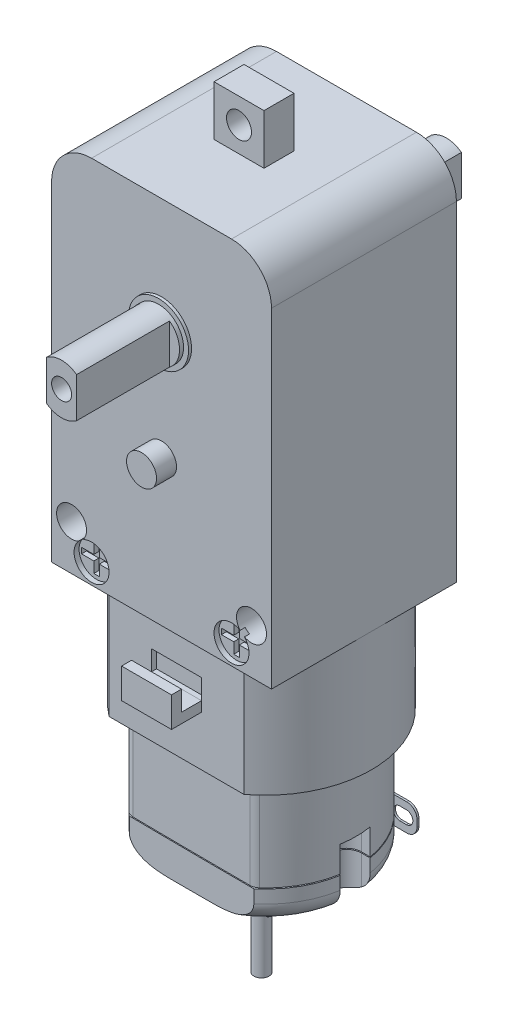
SolidWorks part; units mm, degrees
ref_plane "Front Plane" through (0, 0, 0) normal (0, 0, 1) x (1, 0, 0)
ref_plane "Top Plane" through (0, 0, 0) normal (0, 1, 0) x (1, 0, 0)
ref_plane "Right Plane" through (0, 0, 0) normal (1, 0, 0) x (0, 0, -1)
sketch "Sketch1" plane through (0, 0, 0) normal (0, 0, 1) x (1, 0, 0)
  line L1 (-11, 24.5) -> (11, 24.5)
  line L2 (-11, 24.5) -> (-11, -24.5)
  line L3 (-11, -24.5) -> (11, -24.5)
  line L4 (11, 24.5) -> (11, -24.5)
  line L5 (-11, 24.5) -> (11, -24.5) construction
  line L6 (-11, -24.5) -> (11, 24.5) construction
  point P0 (0, 0)
  dimension "D1" = 22
  dimension "D2" = 49
extrude "Boss-Extrude1" add sketch "Sketch1" along normal mid plane 18.5
sketch "Sketch2" plane through (0, 0, 0) normal (0, 0, 1) x (1, 0, 0)
  line L0 (11, 24.5) -> (-11, 24.5) construction
  line L1 (-2.5, 29.5) -> (2.5, 29.5)
  line L2 (-2.5, 29.5) -> (-2.5, 19.5)
  line L3 (-2.5, 19.5) -> (2.5, 19.5)
  line L4 (2.5, 29.5) -> (2.5, 19.5)
  line L5 (-2.5, 29.5) -> (2.5, 19.5) construction
  line L6 (-2.5, 19.5) -> (2.5, 29.5) construction
  line L7 (-2.5, 29.5) -> (2.5, 24.5) construction
  circle A0 centre (0, 27) radius 1.25
  point P0 (0, 24.5)
  dimension "D3" = 2.5
  dimension "D1" = 5
  dimension "D2" = 10
extrude "Boss-Extrude2" add sketch "Sketch2" along normal blind 1.5 and the other way blind 1.5
fillet "Filete1" radius 4 2 edges at (11, 24.5, 0) (-11, 24.5, 0)
sketch "Sketch4" plane through (0, 0, 9.25) normal (0, 0, 1) x (1, 0, 0)
  line L0 (7, 24.5) -> (-7, 24.5) construction
  circle A0 centre (0, 2) radius 1.5
  dimension "D2" = 3
  dimension "D1" = 24
extrude "Boss-Extrude3" add sketch "Sketch4" along normal blind 2
sketch "Sketch5" plane through (0, -24.5, 0) normal (0, -1, 0) x (1, 0, 0)
  line L0 (-11, 7.75) -> (11, 7.75) construction
  line L1 (-11, 9.25) -> (-11, -9.25) construction
  line L2 (11, 9.25) -> (11, -9.25) construction
  line L3 (-11, 9.25) -> (11, 9.25) construction
  line L4 (-11, -0.75) -> (11, -0.75) construction
  line L5 (-6.75, 9.25) -> (-6.75, -9.25) construction
  line L6 (-11, -9.25) -> (11, -9.25) construction
  line L7 (6.75, 9.25) -> (6.75, -9.25) construction
  line L8 (-6.75, 7.75) -> (6.75, 7.75)
  line L9 (-6.75, -9.25) -> (6.75, -9.25)
  arc A0 (-11, -0.75) -> (-6.75, 7.75) centre (-0.375, -0.75) cw
  arc A1 (-11, -0.75) -> (-6.75, -9.25) centre (-0.375, -0.75) ccw
  arc A2 (11, -0.75) -> (6.75, 7.75) centre (0.375, -0.75) ccw
  arc A3 (11, -0.75) -> (6.75, -9.25) centre (0.375, -0.75) cw
  dimension "D1" = 1.5
  dimension "D2" = 10
  dimension "D3" = 6.75
  dimension "D4" = 6.75
extrude "Cut-Extrude1" cut sketch "Sketch5" against normal blind 12 flip side to cut
sketch "Sketch6" plane through (0, -24.5, 0) normal (0, -1, 0) x (1, 0, 0)
  line L2 (-6.75, -9.25) -> (6.75, -9.25)
  line L3 (6.75, 7.75) -> (-6.75, 7.75)
  line L4 (-6.75, -9.25) -> (6.75, -9.25) construction
  line L5 (6.75, 7.75) -> (-6.75, 7.75) construction
  line L6 (-6.2287, -7.75) -> (6.2287, -7.75)
  line L7 (6.2287, 6.25) -> (-6.2287, 6.25)
  arc A2 (-6.75, 7.75) -> (-6.75, -9.25) centre (-0.375, -0.75) ccw
  arc A3 (6.75, -9.25) -> (6.75, 7.75) centre (0.375, -0.75) ccw
  arc A4 (-6.75, 7.75) -> (-6.75, -9.25) centre (-0.375, -0.75) ccw construction
  arc A5 (6.75, -9.25) -> (6.75, 7.75) centre (0.375, -0.75) ccw construction
  arc A6 (6.2287, -7.75) -> (6.2287, 6.25) centre (0.375, -0.75) ccw
  arc A7 (-6.2287, 6.25) -> (-6.2287, -7.75) centre (-0.375, -0.75) ccw
  dimension "D1" = 0
  dimension "D2" = 1.5
extrude "Boss-Extrude4" add sketch "Sketch6" along normal blind 15
sketch "Sketch7" plane through (0, 0, 0) normal (0, 0, 1) x (1, 0, 0)
  line L0 (9.5, -39.5) -> (9.5, -24.5) construction
  line L1 (5.3527, -33.6) -> (13.6473, -33.6)
  line L2 (5.3527, -33.6) -> (5.3527, -33.7)
  line L3 (5.3527, -33.7) -> (13.6473, -33.7)
  line L4 (13.6473, -33.6) -> (13.6473, -33.7)
  line L5 (5.3527, -33.6) -> (13.6473, -33.7) construction
  line L6 (5.3527, -33.7) -> (13.6473, -33.6) construction
  line L7 (6.2287, -24.5) -> (9.5, -24.5) construction
  line L8 (0, 0) -> (-0.375, -57.0989) construction
  point P0 (9.5, -33.65)
  dimension "D1" = 0.1
  dimension "D2" = 9.2
revolve "Cut-Revolve1" cut sketch "Sketch7" angle 360 about L8
sketch "Sketch8" plane through (0, -39.5, 0) normal (0, -1, 0) x (1, 0, 0)
  line L0 (-3.7417, 2.5) -> (3.7417, 2.5)
  arc A0 (-3.7417, 2.5) -> (3.7417, 2.5) centre (0, 0) ccw
  dimension "D1" = 9
  dimension "D2" = 7
extrude "Cut-Extrude2" cut sketch "Sketch8" against normal blind 2.5 flip side to cut
fillet "Filete3" radius 0.5 2 edges at (0, -39.5, -4.5) (0, -39.5, 2.5)
sketch "Sketch9" plane through (0, -37, 0) normal (0, -1, 0) x (1, 0, 0)
  line L0 (-10.5, -0.75) -> (-8.5, -0.75) construction
  line L1 (-10.5, 0.75) -> (-8.5, 0.75)
  line L2 (-10.5, -2.25) -> (-8.5, -2.25)
  line L3 (10.5, -0.75) -> (8.5, -0.75) construction
  line L4 (10.5, -2.25) -> (8.5, -2.25)
  line L5 (10.5, 0.75) -> (8.5, 0.75)
  arc A0 (-6.2287, 6.25) -> (-6.2287, -7.75) centre (-0.375, -0.75) ccw construction
  arc A1 (-10.5, 0.75) -> (-10.5, -2.25) centre (-10.5, -0.75) ccw
  arc A2 (-8.5, -2.25) -> (-8.5, 0.75) centre (-8.5, -0.75) ccw
  arc A3 (6.2287, -7.75) -> (6.2287, 6.25) centre (0.375, -0.75) ccw construction
  arc A4 (10.5, -2.25) -> (10.5, 0.75) centre (10.5, -0.75) ccw
  arc A5 (8.5, 0.75) -> (8.5, -2.25) centre (8.5, -0.75) ccw
  point P6 (-9.5, -0.75)
  point P12 (9.5, -0.75)
  dimension "D1" = 3
  dimension "D2" = 3
  dimension "D3" = 1
  dimension "D4" = 1
extrude "Cut-Extrude3" cut sketch "Sketch9" against normal blind 6
sketch "Sketch10" plane through (0, -39.5, 0) normal (0, -1, 0) x (1, 0, 0)
  line L0 (-11, -0.75) -> (0, -0.75) construction
  circle A0 centre (0, -0.75) radius 0.75
  arc A1 (-6.75, 7.75) -> (-6.75, -9.25) centre (-0.375, -0.75) ccw construction
  dimension "D1" = 1.5
extrude "Boss-Extrude5" add sketch "Sketch10" along normal blind 8 separate body
fillet "Filete4" radius 2 4 edges at (8.295, -37, 3.782) (8.295, -37, -5.282) (-8.295, -37, -5.282) (-8.295, -37, 3.782)
sketch "Sketch11" plane through (0, 0, -7.75) normal (0, 0, -1) x (-1, 0, 0)
  line L0 (0, -33.6505) -> (0, 0) construction
  line L1 (-4.25, -33.6505) -> (4.25, -33.6505)
  line L2 (-4.25, -33.6505) -> (-4.25, -36.6505)
  line L3 (-4.25, -36.6505) -> (4.25, -36.6505)
  line L4 (4.25, -33.6505) -> (4.25, -36.6505)
  line L5 (-4.25, -33.6505) -> (4.25, -36.6505) construction
  line L6 (-4.25, -36.6505) -> (4.25, -33.6505) construction
  spline S0 degree 3 poles (-6.2287, -33.6761) (-4.1524, -33.6712) (-2.0761, -33.6638) (2.0763, -33.6373) (4.1525, -33.6181) (6.2287, -33.5961) knots 0 0 0 0 0.5 0.5 1 1 1 1 construction
  point P0 (0, -35.1505)
  dimension "D1" = 3
  dimension "D2" = 8.5
extrude "Boss-Extrude6" add sketch "Sketch11" along normal blind 2 separate body
sketch "Sketch12" plane through (4.25, 0, 0) normal (1, 0, 0) x (0, 0, -1)
  line L0 (9.15, -35.1505) -> (9.75, -35.1505) construction
  line L1 (9.05, -33.8005) -> (9.25, -33.8005)
  line L2 (9.05, -33.8005) -> (9.05, -36.5005)
  line L3 (9.05, -36.5005) -> (9.25, -36.5005)
  line L4 (9.25, -33.8005) -> (9.25, -36.5005)
  line L5 (9.05, -33.8005) -> (9.25, -36.5005) construction
  line L6 (9.05, -36.5005) -> (9.25, -33.8005) construction
  line L7 (9.75, -33.6505) -> (9.75, -36.6505) construction
  point P0 (9.15, -35.1505)
  dimension "D1" = 0.2
  dimension "D2" = 2.7
  dimension "D3" = 0.5
extrude "Boss-Extrude7" add sketch "Sketch12" along normal blind 3
sketch "Sketch13" plane through (-4.25, 0, 0) normal (-1, 0, 0) x (0, 0, 1)
  line L4 (-9.25, -33.8005) -> (-9.25, -36.5005)
  line L5 (-9.05, -33.8005) -> (-9.25, -33.8005)
  line L6 (-9.05, -36.5005) -> (-9.05, -33.8005)
  line L7 (-9.25, -36.5005) -> (-9.05, -36.5005)
  line L8 (-9.25, -33.8005) -> (-9.25, -36.5005)
  line L9 (-9.05, -33.8005) -> (-9.25, -33.8005)
  line L10 (-9.05, -36.5005) -> (-9.05, -33.8005)
  line L11 (-9.25, -36.5005) -> (-9.05, -36.5005)
  dimension "D1" = 0
extrude "Boss-Extrude8" add sketch "Sketch13" along normal blind 3.5
fillet "Filete5" radius 1 4 edges at (-7.75, -36.5005, -9.15) (-7.75, -33.8005, -9.15) (7.25, -36.5005, -9.15) (7.25, -33.8005, -9.15)
sketch "Sketch14" plane through (0, 0, -9.25) normal (0, 0, -1) x (-1, 0, 0)
  line L0 (-6.199, -35.1505) -> (-5.5372, -35.1505) construction
  line L1 (-6.199, -34.5079) -> (-5.5372, -34.5079)
  line L2 (-6.199, -35.7931) -> (-5.5372, -35.7931)
  line L3 (-7.25, -35.1505) -> (-5.8681, -35.1505) construction
  line L4 (-7.25, -35.5005) -> (-7.25, -34.8005) construction
  line L5 (0, -36.6505) -> (0, -26.142) construction
  line L6 (-4.25, -36.6505) -> (4.25, -36.6505) construction
  line L7 (6.199, -35.1505) -> (5.5372, -35.1505) construction
  line L8 (6.199, -34.5079) -> (5.5372, -34.5079)
  line L9 (6.199, -35.7931) -> (5.5372, -35.7931)
  arc A0 (-6.199, -34.5079) -> (-6.199, -35.7931) centre (-6.199, -35.1505) ccw
  arc A1 (-5.5372, -35.7931) -> (-5.5372, -34.5079) centre (-5.5372, -35.1505) ccw
  arc A2 (6.199, -34.5079) -> (6.199, -35.7931) centre (6.199, -35.1505) cw
  arc A3 (5.5372, -35.7931) -> (5.5372, -34.5079) centre (5.5372, -35.1505) cw
  point P2 (-5.8681, -35.1505)
  point P18 (5.8681, -35.1505)
  dimension "D2" = 0.6426
  dimension "D1" = 1.3819
  dimension "D3" = 0.6618
extrude "Cut-Extrude4" cut sketch "Sketch14" against normal blind 1
sketch "Sketch16" plane through (0, 0, 0) normal (1, 0, 0) x (0, 0, -1)
  line L0 (0.75, -24.5) -> (0.75, -1.0627) construction
  line L2 (-7.75, -24.5) -> (9.25, -24.5) construction
  line L3 (9.25, -19.5) -> (12.25, -19.5)
  line L4 (9.25, -12.5) -> (9.25, -24.5) construction
  line L5 (-7.75, -19.5) -> (-10.75, -19.5)
  line L6 (12.25, -19.5) -> (12.25, -16.5)
  line L7 (-10.75, -19.5) -> (-10.75, -16.5)
  line L8 (12.25, -16.5) -> (11.25, -16.5)
  line L9 (-10.75, -16.5) -> (-9.75, -16.5)
  line L10 (11.25, -16.5) -> (11.25, -18.5)
  line L11 (-9.75, -16.5) -> (-9.75, -18.5)
  line L12 (11.25, -18.5) -> (9.25, -18.5)
  line L13 (-9.75, -18.5) -> (-7.75, -18.5)
  line L14 (9.25, -18.5) -> (9.25, -19.5)
  line L15 (-7.75, -18.5) -> (-7.75, -19.5)
  line L16 (-9.25, 24.5) -> (9.25, 24.5) construction
  dimension "D1" = 44
  dimension "D2" = 41
  dimension "D3" = 1
  dimension "D4" = 3
  dimension "D5" = 1
extrude "Boss-Extrude9" add sketch "Sketch16" along normal mid plane 5 separate body
fillet "Filete6" radius 1 4 edges at (-6.2287, -29.0018, 6.25) (6.2287, -29.0417, 6.25) (-6.2287, -28.9981, -7.75) (6.2287, -29.0381, -7.75)
sketch "Sketch17" plane through (0, 0, -9.25) normal (0, 0, -1) x (-1, 0, 0)
  line L1 (-2.5, -16.5) -> (2.5, -16.5)
  line L2 (-2.5, -16.5) -> (-2.5, -18.5)
  line L3 (-2.5, -18.5) -> (2.5, -18.5)
  line L4 (2.5, -16.5) -> (2.5, -18.5)
extrude "Cut-Extrude5" cut sketch "Sketch17" against normal blind 0.5
sketch "Sketch18" plane through (0, 0, 7.75) normal (0, 0, 1) x (1, 0, 0)
  line L4 (2.5, -16.5) -> (-2.5, -16.5)
  line L5 (-2.5, -16.5) -> (-2.5, -18.5)
  line L6 (-2.5, -18.5) -> (2.5, -18.5)
  line L7 (2.5, -18.5) -> (2.5, -16.5)
  line L8 (2.5, -16.5) -> (-2.5, -16.5)
  line L9 (-2.5, -16.5) -> (-2.5, -18.5)
  line L10 (-2.5, -18.5) -> (2.5, -18.5)
  line L11 (2.5, -18.5) -> (2.5, -16.5)
  dimension "D1" = 0
extrude "Cut-Extrude6" cut sketch "Sketch18" against normal blind 0.5
sketch "Sketch19" plane through (0, 0, 9.25) normal (0, 0, 1) x (1, 0, 0)
  line L3 (6.75, -12.5) -> (11, -12.5) construction
  line L4 (-9, -8) -> (9, -8) construction
  line L5 (0, -8) -> (0, -12.5) construction
  line L6 (6.75, -12.5) -> (-6.75, -12.5) construction
  circle A0 centre (-9, -8) radius 1.5
  circle A1 centre (9, -8) radius 1.5
  dimension "D1" = 15
  dimension "D2" = 3
  dimension "D3" = 3
  dimension "D4" = 3
extrude "Cut-Extrude7" cut sketch "Sketch19" against normal through all
sketch "Sketch20" plane through (0, 0, 9.25) normal (0, 0, 1) x (1, 0, 0)
  line L0 (-7, -10.5) -> (7, -10.5) construction
  line L1 (0, -10.5) -> (0, -12.5) construction
  line L2 (6.75, -12.5) -> (-6.75, -12.5) construction
  line L3 (-11, -12.5) -> (11, -12.5) construction
  circle A0 centre (-7, -10.5) radius 1.75
  circle A1 centre (7, -10.5) radius 1.75
  dimension "D1" = 3.5
  dimension "D2" = 14
  dimension "D3" = 2
extrude "Cut-Extrude8" cut sketch "Sketch20" against normal blind 0.5
sketch "Sketch21" plane through (0, 0, 8.75) normal (0, 0, 1) x (1, 0, 0)
  line L0 (0, -12.5) -> (0, -4.5748) construction
  line L1 (-11, -12.5) -> (11, -12.5) construction
  line L2 (7.2744, -9.1335) -> (7.2744, -11.8665)
  line L3 (-7.2744, -9.1335) -> (-6.7256, -9.1335)
  line L4 (-7.2744, -9.1335) -> (-7.2744, -10.2167)
  line L5 (-7.2744, -11.8665) -> (-6.7256, -11.8665)
  line L6 (-6.7256, -9.1335) -> (-6.7256, -10.2167)
  line L9 (7.2744, -9.1335) -> (6.7256, -11.8665) construction
  line L10 (7.2744, -11.8665) -> (6.7256, -9.1335) construction
  line L11 (7.2744, -9.1335) -> (6.7256, -9.1335)
  line L12 (6.7256, -9.1335) -> (6.7256, -11.8665)
  line L13 (7.2744, -11.8665) -> (6.7256, -11.8665)
  line L14 (8.5048, -10.7833) -> (8.5048, -10.2167)
  line L15 (-8.5048, -10.7833) -> (-7.2744, -10.7833)
  line L16 (-8.5048, -10.7833) -> (-8.5048, -10.2167)
  line L17 (-8.5048, -10.2167) -> (-7.2744, -10.2167)
  line L18 (-5.4952, -10.7833) -> (-5.4952, -10.2167)
  line L21 (8.5048, -10.7833) -> (5.4952, -10.2167) construction
  line L22 (8.5048, -10.2167) -> (5.4952, -10.7833) construction
  line L23 (8.5048, -10.7833) -> (5.4952, -10.7833)
  line L24 (5.4952, -10.7833) -> (5.4952, -10.2167)
  line L25 (8.5048, -10.2167) -> (5.4952, -10.2167)
  line L28 (-7.2744, -10.7833) -> (-7.2744, -11.8665)
  line L30 (-6.7256, -10.7833) -> (-5.4952, -10.7833)
  line L31 (-6.7256, -10.7833) -> (-6.7256, -11.8665)
  line L33 (-6.7256, -10.2167) -> (-5.4952, -10.2167)
  point P5 (-7, -10.5)
  point P14 (7, -10.5)
  point P16 (-7, -10.5)
extrude "Cut-Extrude9" cut sketch "Sketch21" against normal blind 0.5 contours L33 L6 L3 L4 L17 L16 L15 L28 L5 L31 L30 L18 | L12 L25 L24 L23 | L25 L2 L11 L12 | L14 L25 L2 L23 | L2 L23 L12 L13 | L2 L25 L12 L23
sketch "Sketch23" plane through (0, 0, 9.25) normal (0, 0, 1) x (1, 0, 0)
  line L0 (7, 24.5) -> (-7, 24.5) construction
  line L1 (0, 24.5) -> (0, 13) construction
  line L2 (2.5, 24.5) -> (-2.5, 24.5) construction
  circle A0 centre (0, 13) radius 2.5
  dimension "D1" = 5
  dimension "D2" = 14
extrude "Boss-Extrude10" add sketch "Sketch23" along normal blind 10 separate body
sketch "Sketch24" plane through (0, 0, 9.25) normal (0, 0, 1) x (1, 0, 0)
  circle A0 centre (0, 13) radius 2.5 construction
  circle A1 centre (0, 13) radius 2.5
  circle A2 centre (0, 13) radius 3
  dimension "D1" = 6
extrude "Boss-Extrude11" add sketch "Sketch24" along normal blind 0.3 separate body
sketch "Sketch25" plane through (0, 0, -9.25) normal (0, 0, -1) x (-1, 0, 0)
  circle A1 centre (0, 13) radius 2.5
  circle A2 centre (0, 13) radius 2.5
  dimension "D1" = 0
extrude "Boss-Extrude12" add sketch "Sketch25" along normal blind 10
sketch "Sketch26" plane through (0, 0, -9.25) normal (0, 0, -1) x (-1, 0, 0)
  circle A0 centre (0, 13) radius 2.5 construction
  circle A1 centre (0, 13) radius 3
  circle A2 centre (0, 13) radius 3
  circle A3 centre (0, 13) radius 2.5
  dimension "D1" = 0
extrude "Boss-Extrude13" add sketch "Sketch26" along normal blind 0.3 separate body
sketch "Sketch27" plane through (0, 0, 19.25) normal (0, 0, 1) x (1, 0, 0)
  line L1 (-1.5, 18.6212) -> (1.5, 18.6212)
  line L2 (-1.5, 18.6212) -> (-1.5, 7.3788)
  line L3 (-1.5, 7.3788) -> (1.5, 7.3788)
  line L4 (1.5, 18.6212) -> (1.5, 7.3788)
  line L5 (-1.5, 18.6212) -> (1.5, 7.3788) construction
  line L6 (-1.5, 7.3788) -> (1.5, 18.6212) construction
  circle A0 centre (0, 13) radius 1
  point P0 (0, 13)
  dimension "D2" = 2
  dimension "D1" = 3
extrude "Cut-Extrude10" cut sketch "Sketch27" against normal blind 9.3 flip side to cut
sketch "Sketch28" plane through (0, 0, -19.25) normal (0, 0, -1) x (-1, 0, 0)
  line L4 (1.5, 18.6212) -> (-1.5, 18.6212)
  line L5 (-1.5, 18.6212) -> (-1.5, 7.3788)
  line L6 (-1.5, 7.3788) -> (1.5, 7.3788)
  line L7 (1.5, 7.3788) -> (1.5, 18.6212)
  line L8 (1.5, 18.6212) -> (-1.5, 18.6212)
  line L9 (-1.5, 18.6212) -> (-1.5, 7.3788)
  line L10 (-1.5, 7.3788) -> (1.5, 7.3788)
  line L11 (1.5, 7.3788) -> (1.5, 18.6212)
  circle A1 centre (0, 13) radius 1
  circle A2 centre (0, 13) radius 1
  dimension "D1" = 0
  dimension "D2" = 0
extrude "Cut-Extrude11" cut sketch "Sketch28" against normal blind 9.3 flip side to cut
